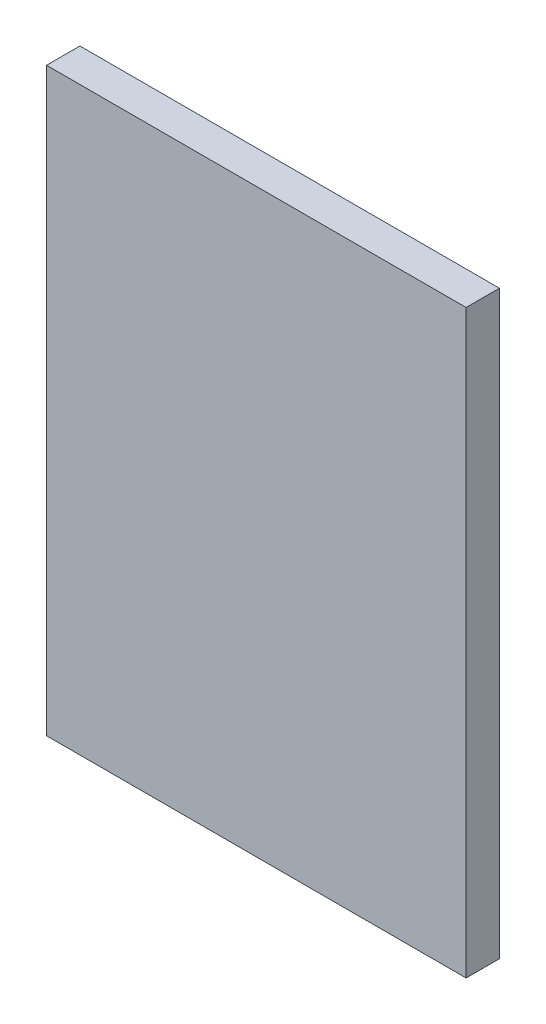
SolidWorks part; units mm, degrees
material "1023 碳钢板 (SS)"
ref_plane "前视基准面" through (0, 0, 0) normal (0, 0, 1) x (1, 0, 0)
ref_plane "上视基准面" through (0, 0, 0) normal (0, 1, 0) x (1, 0, 0)
ref_plane "右视基准面" through (0, 0, 0) normal (1, 0, 0) x (0, 0, -1)
sketch "草图1" plane through (0, 0, 0) normal (0, 0, 1) x (1, 0, 0)
  line L1 (75.5, 104.5) -> (-75.5, 104.5)
  line L2 (75.5, 104.5) -> (75.5, -104.5)
  line L3 (75.5, -104.5) -> (-75.5, -104.5)
  line L4 (-75.5, 104.5) -> (-75.5, -104.5)
  line L5 (75.5, 104.5) -> (-75.5, -104.5) construction
  line L6 (75.5, -104.5) -> (-75.5, 104.5) construction
  point P0 (0, 0)
  dimension "D1" = 151
  dimension "D2" = 209
extrude "凸台-拉伸1" add sketch "草图1" along normal blind 12
